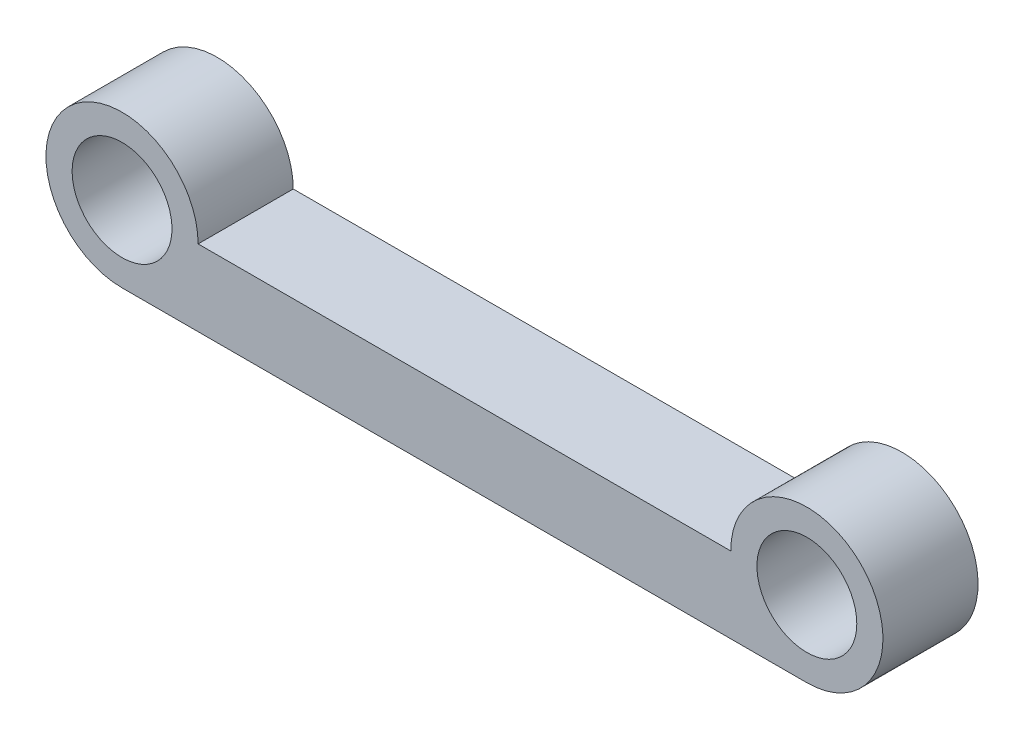
SolidWorks part; units mm, degrees
ref_plane "Front Plane" through (0, 0, 0) normal (0, 0, 1) x (1, 0, 0)
ref_plane "Top Plane" through (0, 0, 0) normal (0, 1, 0) x (1, 0, 0)
ref_plane "Right Plane" through (0, 0, 0) normal (1, 0, 0) x (0, 0, -1)
other "Configuration Table"
sketch "Sketch1" plane through (0, 0, 0) normal (0, 0, 1) x (1, 0, 0)
  line L1 (-17.5, -2.5) -> (17.5, -2.5)
  line L2 (-17.5, -2.5) -> (-17.5, 2.5)
  line L3 (-17.5, 2.5) -> (17.5, 2.5)
  line L4 (17.5, -2.5) -> (17.5, 2.5)
  line L5 (-17.5, -2.5) -> (17.5, 2.5) construction
  line L6 (-17.5, 2.5) -> (17.5, -2.5) construction
  point P0 (0, 0)
  dimension "D1" = 35
  dimension "D2" = 5
extrude "Boss-Extrude3" add sketch "Sketch1" along normal blind 5 contours L3 L4 L1 L2
sketch "Sketch4" plane through (0, 0, 5) normal (0, 0, 1) x (1, 0, 0)
  line L0 (17.5, 0) -> (16, 0) construction
  line L1 (17.5, -2.5) -> (17.5, 2.5) construction
  line L2 (16, 0) -> (17.5, 0) construction
  line L3 (17.5, 0) -> (16, 0) construction
  circle A0 centre (16, 0) radius 1
sketch "Sketch5" plane through (0, 0, 5) normal (0, 0, 1) x (1, 0, 0)
  line L0 (-17.5, 0) -> (-16, 0) construction
  line L1 (-17.5, -2.5) -> (-17.5, 2.5) construction
  line L2 (-16, 0) -> (-17.5, 0) construction
  line L3 (-17.5, 0) -> (-16, 0) construction
  circle A0 centre (-16, 0) radius 2.375
sketch "Sketch7" plane through (0, 0, 5) normal (0, 0, 1) x (1, 0, 0)
  line L0 (22.5, -2.4538) -> (17.5, -2.4538)
  line L5 (22.5, -2.4538) -> (22.5, 2.5462)
  line L6 (17.5, -2.4538) -> (17.5, 2.5462)
  line L7 (22.5, 2.5462) -> (17.5, 2.5462)
  line L8 (22.5, -2.4538) -> (17.5, 2.5462) construction
  line L9 (17.5, -2.4538) -> (22.5, 2.5462) construction
  point P1 (20, 0.0462)
extrude "Boss-Extrude6" add sketch "Sketch7" against normal blind 5
fillet "Fillet6" radius 1 1 edges at (22.5, 2.5462, 2.5)
fillet "Fillet7" radius 1 1 edges at (22.5, -2.4538, 2.5)
sketch "Sketch11" plane through (0, 0, 5) normal (0, 0, 1) x (1, 0, 0)
  line L0 (17.5, 0) -> (22.5, 0.0462) construction
  line L1 (22.5, -1.4538) -> (22.5, 1.5462) construction
  circle A0 centre (20, 0.0231) radius 2
extrude "Cut-Extrude2" cut sketch "Sketch11" against normal blind 5
sketch "Sketch12" plane through (-17.5, 0, 0) normal (-1, 0, 0) x (0, 0, 1)
  line L1 (0, 2.5) -> (4, 2.5)
  line L2 (0, 2.5) -> (0, -1.5)
  line L3 (0, -1.5) -> (4, -1.5)
  line L4 (4, 2.5) -> (4, -1.5)
extrude "Boss-Extrude9" add sketch "Sketch5" along normal blind 5
sketch "Sketch13" plane through (0, 0, 5) normal (0, 0, 1) x (1, 0, 0)
  circle A0 centre (20, 0.0231) radius 4
extrude "Boss-Extrude10" add sketch "Sketch13" against normal through all
sketch "Sketch14" plane through (0, 0, 5) normal (0, 0, 1) x (1, 0, 0)
  circle A0 centre (20, 0.0231) radius 2.625
extrude "Cut-Extrude3" cut sketch "Sketch14" against normal through all
sketch "Sketch15" plane through (-17.5, 0, 0) normal (-1, 0, 0) x (0, 0, 1)
  line L1 (0, 2.5) -> (5, 2.5)
  line L2 (0, 2.5) -> (0, -2.5)
  line L3 (0, -2.5) -> (5, -2.5)
  line L4 (5, 2.5) -> (5, -2.5)
extrude "Boss-Extrude11" add sketch "Sketch15" along normal through all
fillet "Fillet8" radius 2 1 edges at (-18.375, 2.5, 2.5)
fillet "Fillet9" radius 2 1 edges at (-18.375, -2.5, 2.5)
sketch "Sketch16" plane through (0, 0, 5) normal (0, 0, 1) x (1, 0, 0)
  circle A0 centre (-16, 0) radius 4
extrude "Boss-Extrude12" add sketch "Sketch16" against normal blind 5
sketch "Sketch17" plane through (0, 0, 10) normal (0, 0, 1) x (1, 0, 0)
  circle A0 centre (-16, 0) radius 2.625
extrude "Cut-Extrude4" cut sketch "Sketch17" against normal blind 30
sketch "Sketch18" plane through (0, 0, 5) normal (0, 0, 1) x (1, 0, 0)
  line L0 (-12, 0) -> (16, 0.0231)
  line L1 (-16, 4) -> (19.9974, 4.0231)
  arc A0 (-12, 0) -> (-16, 4) centre (-16, 0) ccw
  arc A1 (19.9974, 4.0231) -> (16, 0.0231) centre (20, 0.0231) ccw
extrude "Cut-Extrude5" cut sketch "Sketch18" against normal through all
sketch "Sketch19" plane through (0, 0, 5) normal (0, 0, 1) x (1, 0, 0)
  line L0 (-16, -4) -> (20, -3.9769)
  line L1 (20, -3.9769) -> (16, -1.2733)
  line L2 (16, -1.2733) -> (-12.8786, -1.6492)
  line L3 (-12.8786, -1.6492) -> (-16, -4)
  arc A0 (-12, 0) -> (-12.8775, -2.5) centre (-16, 0) ccw construction
  arc A1 (16.8961, -2.5) -> (16, 0.0231) centre (20, 0.0231) ccw construction
extrude "Boss-Extrude13" add sketch "Sketch19" against normal through all
